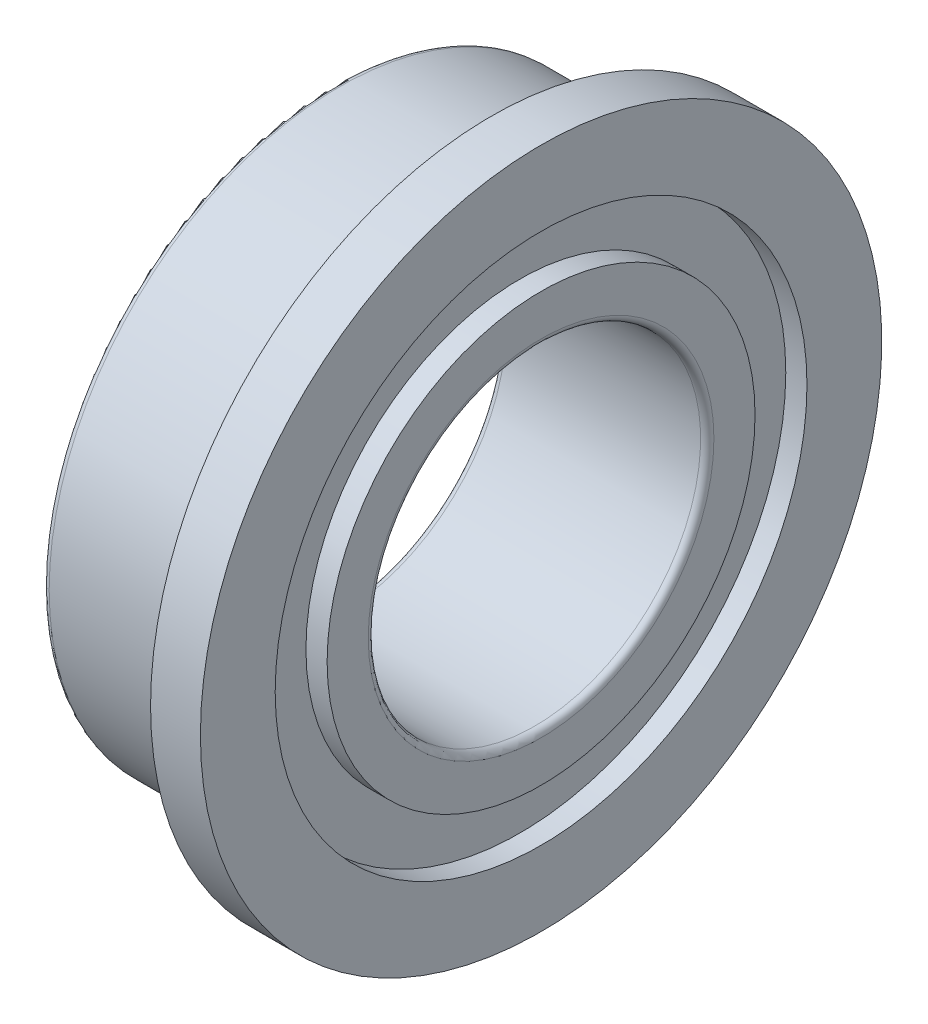
from build123d import *


with BuildPart() as part:
    # Sketch1 → Revolve1 (revolve)
    with BuildSketch(Plane.XY, mode=Mode.PRIVATE) as revolve1_sk:
        with BuildLine():
            Line((0, 3.42), (0, 3.2))
            Line((0, 3.2), (0.255, 3.2))
            Line((0.255, 3.2), (0.255, 2.575))
            Line((0.255, 2.575), (0, 2.575))
            Line((0, 2.575), (0, 2.08))
            ThreePointArc((0, 2.08), (0.023431458, 2.023431458), (0.08, 2))
            Line((0.08, 2), (2.42, 2))
            ThreePointArc((2.42, 2), (2.476568542, 2.023431458), (2.5, 2.08))
            Line((2.5, 2.08), (2.5, 2.575))
            Line((2.5, 2.575), (2.245, 2.575))
            Line((2.245, 2.575), (2.245, 3.2))
            Line((2.245, 3.2), (2.5, 3.2))
            Line((2.5, 3.2), (2.5, 4.1))
            Line((2.5, 4.1), (1.9, 4.1))
            Line((1.9, 4.1), (1.9, 3.58))
            ThreePointArc((1.9, 3.58), (1.956568542, 3.443431458), (1.82, 3.5))
            Line((1.82, 3.5), (0.08, 3.5))
            ThreePointArc((0.08, 3.5), (0.023431458, 3.476568542), (0, 3.42))
        make_face()
    revolve(revolve1_sk.sketch.rotate(Axis((7, 0, 0), (-1, 0, 0)), 270), axis=Axis((7, 0, 0), (-1, 0, 0)))


solid = part.part
